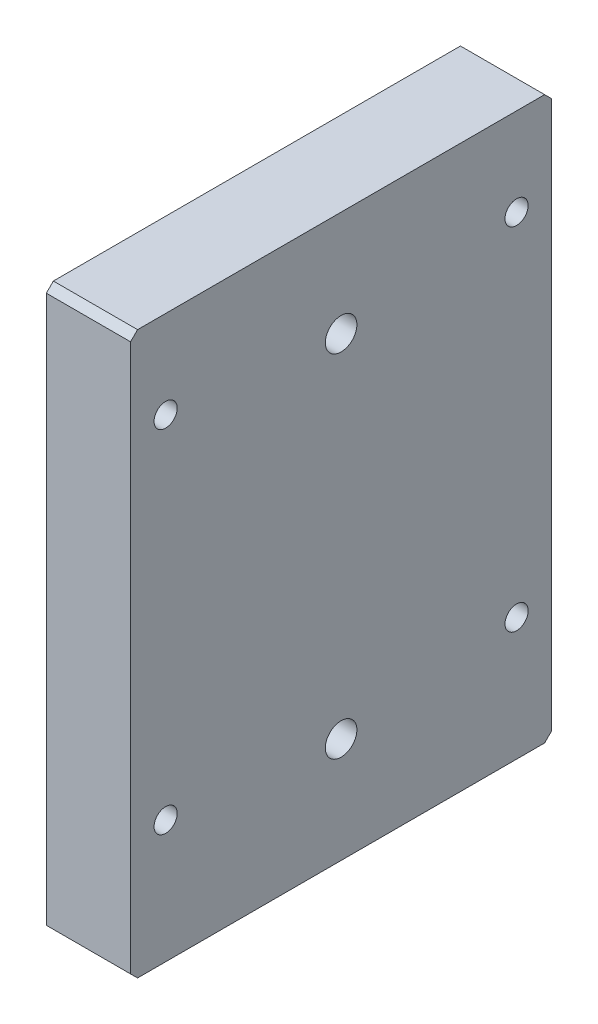
from build123d import *

# Parameters (mm, degrees)
SKETCH1_W                                            = 60
SKETCH1_H                                            = 80
BOSS_EXTRUDE1_DEPTH                                  = 12
M4_TAPPED_HOLE1_D                                    = 3.3
CBORE_FOR_M4_HEXAGON_SOCKET_HEAD_CAP_SCR_D           = 4.5
CBORE_FOR_M4_HEXAGON_SOCKET_HEAD_CAP_SCR_CBORE_D     = 8
CBORE_FOR_M4_HEXAGON_SOCKET_HEAD_CAP_SCR_CBORE_DEPTH = 4.6
CHAMFER1_SIZE                                        = 1


with BuildPart() as part:
    # Sketch1 → Boss-Extrude1 (new body)
    with BuildSketch(Plane(origin=(0, 0, 0), x_dir=(0, 0, -1), z_dir=(1, 0, 0))):
        Rectangle(SKETCH1_W, SKETCH1_H)
    extrude(amount=BOSS_EXTRUDE1_DEPTH)

    # M4 Tapped Hole1 (through all)
    with Locations(Plane.ZY):
        with Locations((-25, 27.5), (-25, -22.5), (25, -22.5), (25, 27.5)):
            Hole(M4_TAPPED_HOLE1_D / 2)

    # CBORE for M4 Hexagon socket head cap screws1 (through all)
    with Locations(Plane.ZY):
        with Locations((0, -25), (0, 25)):
            CounterBoreHole(CBORE_FOR_M4_HEXAGON_SOCKET_HEAD_CAP_SCR_D / 2, CBORE_FOR_M4_HEXAGON_SOCKET_HEAD_CAP_SCR_CBORE_D / 2, CBORE_FOR_M4_HEXAGON_SOCKET_HEAD_CAP_SCR_CBORE_DEPTH)

    # Chamfer1
    chamfer1_edges = [part.edges().sort_by_distance(p)[0] for p in [
        (6, -40, -30),
        (6, -40, 30),
        (6, 40, 30),
        (6, 40, -30),
    ]]
    chamfer(chamfer1_edges, length=CHAMFER1_SIZE)


solid = part.part
